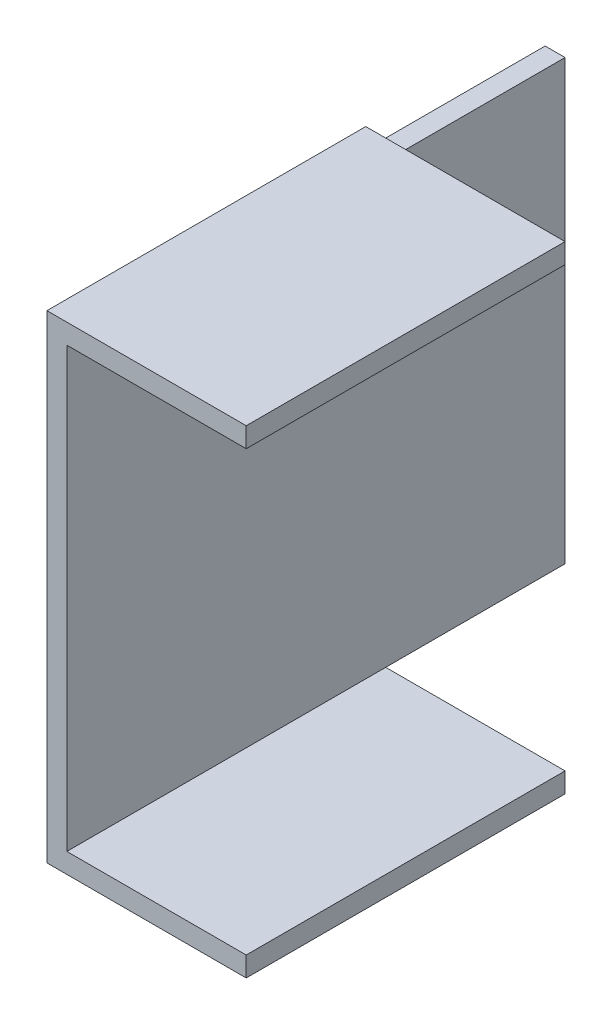
from build123d import *

# Parameters (mm, degrees)
EXTRUDE_1_DEPTH     = 150
SKETCH_2_W          = 50
SKETCH_2_H          = 5
CUT_EXTRUDE_1_DEPTH = 45
SKETCH_3_W          = 5
SKETCH_3_H          = 110
CUT_EXTRUDE_2_DEPTH = 25
CUT_EXTRUDE_3_DEPTH = 25
CUT_EXTRUDE_4_DEPTH = 25


with BuildPart() as part:
    # 草图1 → 凸台-拉伸1 (new body)
    with BuildSketch(Plane.XY):
        Polygon((0, 0), (0, 120), (50, 120), (50, 115), (5, 115), (5, 5), (50, 5), (50, 0), align=None)
    extrude(amount=-EXTRUDE_1_DEPTH)

    # 草图2 → 切除-拉伸1 (cut)
    with BuildSketch(Plane(origin=(0, 0, -150), x_dir=(-1, 0, 0), z_dir=(0, 0, -1))):
        with Locations((-25, 117.5)):
            Rectangle(SKETCH_2_W, SKETCH_2_H)
        with Locations((-25, 2.5)):
            Rectangle(SKETCH_2_W, SKETCH_2_H)
    extrude(amount=-CUT_EXTRUDE_1_DEPTH, mode=Mode.SUBTRACT)

    # 草图3 → 切除-拉伸2 (cut)
    with BuildSketch(Plane(origin=(0, 0, -150), x_dir=(-1, 0, 0), z_dir=(0, 0, -1))):
        with Locations((-2.5, 60)):
            Rectangle(SKETCH_3_W, SKETCH_3_H)
    extrude(amount=-CUT_EXTRUDE_2_DEPTH, mode=Mode.SUBTRACT)

    # 草图4 → 切除-拉伸3 (cut)
    with BuildSketch(Plane(origin=(0, 0, -105), x_dir=(-1, 0, 0), z_dir=(0, 0, -1))):
        Polygon((-50, 120), (-50, 115), (-5, 115), (0, 115), (0, 120), align=None)
    extrude(amount=-CUT_EXTRUDE_3_DEPTH, mode=Mode.SUBTRACT)

    # 草图5 → 切除-拉伸4 (cut)
    with BuildSketch(Plane(origin=(0, 0, -105), x_dir=(-1, 0, 0), z_dir=(0, 0, -1))):
        Polygon((-50, 5), (-50, 0), (0, 0), (0, 5), (-5, 5), align=None)
    extrude(amount=-CUT_EXTRUDE_4_DEPTH, mode=Mode.SUBTRACT)


solid = part.part
